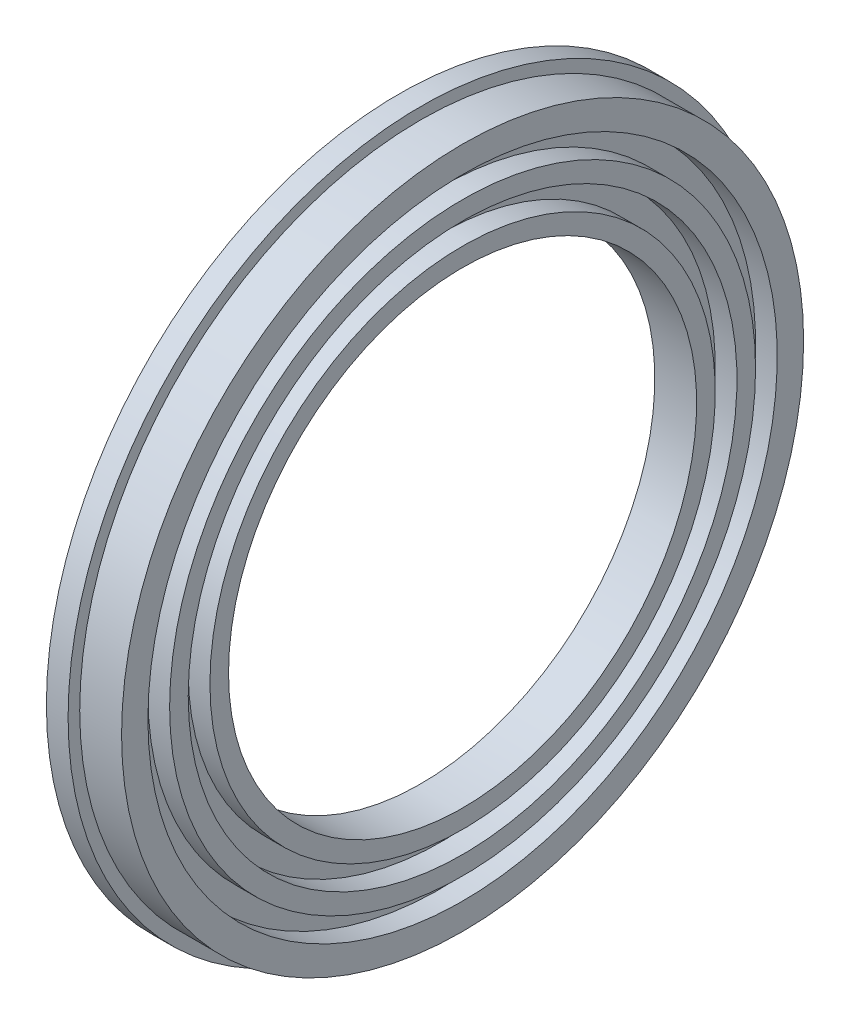
from build123d import *

# Parameters (mm, degrees)
FILLET1_R = 10


with BuildPart() as part:
    # Sketch1 → Revolve1 (revolve)
    with BuildSketch(Plane(origin=(0, 0, 0), x_dir=(1, 0, 0), z_dir=(0, 1, 0)), mode=Mode.PRIVATE) as revolve1_sk:
        Polygon((0, 200), (0, 227.5), (14, 227.5), (14, 220), (41, 220), (41, 203), (27, 203), (27, 189), (41, 189), (41, 177), (27, 177), (27, 163), (41, 163), (41, 151), (14, 151), (14, 200), align=None)
    revolve(revolve1_sk.sketch.rotate(Axis((0, 0, 0), (1, 0, 0)), 180), axis=Axis((0, 0, 0), (1, 0, 0)))

    # Fillet1
    fillet1_edges = [part.edges().sort_by_distance(p)[0] for p in [
        (14, 0, -200),
    ]]
    fillet(fillet1_edges, radius=FILLET1_R)


solid = part.part
